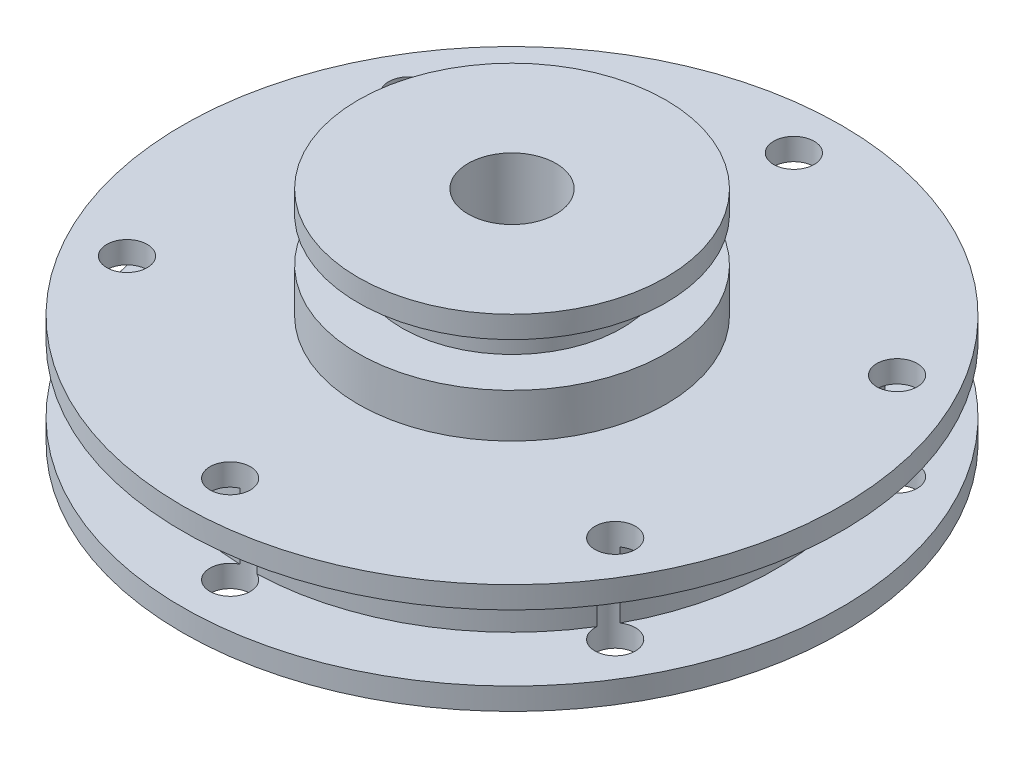
from build123d import *

# Parameters (mm, degrees)
SKETCH1_R               = 15
BOSS_EXTRUDE1_DEPTH     = 5
SKETCH2_W               = 3
SKETCH2_H               = 3
SKETCH3_R               = 7
BOSS_EXTRUDE2_DEPTH     = 5
SKETCH4_W               = 2
SKETCH4_H               = 2
SKETCH5_R               = 2
CUT_EXTRUDE1_DEPTH      = 24.452078799
CUT_EXTRUDE2_DEPTH      = 22.794494718
CUT_EXTRUDE2_DEPTH_BACK = 22.794494718
SKETCH6_R               = 0.920579976


with BuildPart() as part:
    # Sketch1 → Boss-Extrude1 (new body)
    with BuildSketch(Plane(origin=(0, 0, 0), x_dir=(1, 0, 0), z_dir=(0, 1, 0))):
        with Locations(Location((0, 0, 0), (0, 0, 270))):
            Circle(SKETCH1_R)
    extrude(amount=BOSS_EXTRUDE1_DEPTH)

    # Sketch2 → Cut-Revolve1 (revolve, cut)
    with BuildSketch(Plane.XY, mode=Mode.PRIVATE) as cut_revolve1_sk:
        with Locations((13.5, 2.5)):
            Rectangle(SKETCH2_W, SKETCH2_H)
    revolve(cut_revolve1_sk.sketch.rotate(Axis((0, 0, 0), (0, 1, 0)), 90), axis=Axis((0, 0, 0), (0, 1, 0)), mode=Mode.SUBTRACT)

    # Sketch3 → Boss-Extrude2 (add)
    with BuildSketch(Plane(origin=(0, 5, 0), x_dir=(1, 0, 0), z_dir=(0, 1, 0))):
        with Locations(Location((0, 0, 0), (0, 0, 270))):
            Circle(SKETCH3_R)
    extrude(amount=BOSS_EXTRUDE2_DEPTH)

    # Sketch4 → Cut-Revolve2 (revolve, cut)
    with BuildSketch(Plane.XY, mode=Mode.PRIVATE) as cut_revolve2_sk:
        with Locations((6, 8)):
            Rectangle(SKETCH4_W, SKETCH4_H)
    revolve(cut_revolve2_sk.sketch.rotate(Axis((0, 0, 0), (0, 1, 0)), 90), axis=Axis((0, 0, 0), (0, 1, 0)), mode=Mode.SUBTRACT)

    # Sketch5 → Cut-Extrude1 (cut, through all)
    with BuildSketch(Plane(origin=(0, 10, 0), x_dir=(1, 0, 0), z_dir=(0, 1, 0))):
        with Locations(Location((0, 0, 0), (0, 0, 270))):
            Circle(SKETCH5_R)
    extrude(amount=-CUT_EXTRUDE1_DEPTH, mode=Mode.SUBTRACT)

    # Sketch6 → Cut-Extrude2 (cut, two sides: drawn at the far end of the back side and taken through both)
    with BuildSketch(Plane(origin=(0, 5, 0), x_dir=(1, 0, 0), z_dir=(0, 1, 0)).offset(-CUT_EXTRUDE2_DEPTH_BACK)):
        with Locations(Location((0, 12.829886063, 0), (0, 0, 270))):
            Circle(SKETCH6_R)
        with Locations(Location((11.111007258, 6.414943031, 0), (0, 0, 270))):
            Circle(SKETCH6_R)
        with Locations(Location((11.111007258, -6.414943031, 0), (0, 0, 270))):
            Circle(SKETCH6_R)
        with Locations(Location((0, -12.829886063, 0), (0, 0, 270))):
            Circle(SKETCH6_R)
        with Locations(Location((-11.111007258, -6.414943031, 0), (0, 0, 270))):
            Circle(SKETCH6_R)
        with Locations(Location((-11.111007258, 6.414943031, 0), (0, 0, 270))):
            Circle(SKETCH6_R)
    extrude(amount=CUT_EXTRUDE2_DEPTH + CUT_EXTRUDE2_DEPTH_BACK, mode=Mode.SUBTRACT)


solid = part.part
